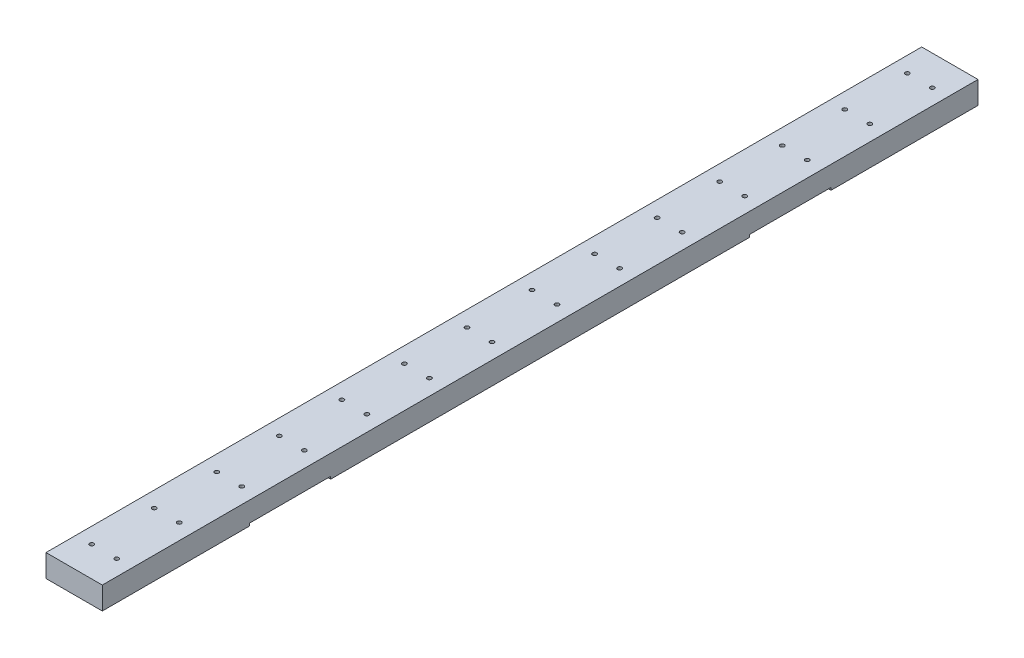
SolidWorks part; units mm, degrees
material "6061-T6"
ref_plane "Front Plane" through (0, 0, 0) normal (0, 0, 1) x (1, 0, 0)
ref_plane "Top Plane" through (0, 0, 0) normal (0, 1, 0) x (1, 0, 0)
ref_plane "Right Plane" through (0, 0, 0) normal (1, 0, 0) x (0, 0, -1)
sketch "Sketch1" plane through (0, 0, 0) normal (0, 0, 1) x (1, 0, 0)
  line L1 (-22.5, 9) -> (22.5, 9)
  line L2 (-22.5, 9) -> (-22.5, -9)
  line L3 (-22.5, -9) -> (22.5, -9)
  line L4 (22.5, 9) -> (22.5, -9)
  line L5 (-22.5, 9) -> (22.5, -9) construction
  line L6 (-22.5, -9) -> (22.5, 9) construction
  point P0 (0, 0)
  dimension "D1" = 45
  dimension "D2" = 18
extrude "Boss-Extrude1" add sketch "Sketch1" along normal mid plane 700
hole_wizard "M4 Tapped Hole1" positions "Sketch2" profile "Sketch3" tap size "M4" standard "GB"
sketch "Sketch2" plane through (-22.5, 0, 0) normal (-1, 0, 0) x (0, 0, 1)
  line L0 (-345, 0) -> (-350, 0)
  line L1 (-350, 9) -> (-350, -9) construction
  line L2 (-345, 0) -> (-300, 0)
  line L3 (300, 0) -> (345, 0)
  point P0 (-345, 0)
  point P19 (-300, 0)
  point P33 (-250, 0)
  point P34 (-200, 0)
  point P35 (-150, 0)
  point P36 (-100, 0)
  point P37 (-50, 0)
  point P38 (0, 0)
  point P39 (50, 0)
  point P40 (100, 0)
  point P41 (150, 0)
  point P42 (200, 0)
  point P43 (250, 0)
  point P44 (300, 0)
  point P46 (345, 0)
  dimension "D1" = 5
  dimension "D2" = 45
  dimension "D4" = 50
  dimension "D5" = 45
  dimension "D3" = 13
sketch "Sketch3" plane through (-22.5, 0, -345) normal (0, 1, 0) x (0, 0, 1)
  line L0 (0, 0) -> (0, 11.0914)
  line L1 (0, 11.0914) -> (1.65, 10.1)
  line L2 (1.65, 10.1) -> (1.65, 0)
  line L5 (1.65, 0) -> (0, 0)
  line L10 (0, 11.0914) -> (-1.65, 10.1) construction
  line L11 (0, -6.35) -> (0, 107.95) construction
  dimension "螺纹孔钻头直径" = 3.3
  dimension "螺纹孔钻头深度" = 10.1
  dimension "导头角度" = 118
cosmetic thread "Hole Thread1" parameters "D1"=8, "D2"=4
cosmetic thread "Hole Thread55" parameters "D1"=8, "D2"=4
cosmetic thread "Hole Thread56" parameters "D1"=8, "D2"=4
cosmetic thread "Hole Thread57" parameters "D1"=8, "D2"=4
cosmetic thread "Hole Thread58" parameters "D1"=8, "D2"=4
cosmetic thread "Hole Thread59" parameters "D1"=8, "D2"=4
cosmetic thread "Hole Thread60" parameters "D1"=8, "D2"=4
cosmetic thread "Hole Thread61" parameters "D1"=8, "D2"=4
cosmetic thread "Hole Thread62" parameters "D1"=8, "D2"=4
cosmetic thread "Hole Thread63" parameters "D1"=8, "D2"=4
cosmetic thread "Hole Thread64" parameters "D1"=8, "D2"=4
cosmetic thread "Hole Thread65" parameters "D1"=8, "D2"=4
cosmetic thread "Hole Thread66" parameters "D1"=8, "D2"=4
cosmetic thread "Hole Thread67" parameters "D1"=8, "D2"=4
cosmetic thread "Hole Thread68" parameters "D1"=8, "D2"=4
pattern_linear "LPattern1" count 14 spacing 50
cosmetic thread "Hole Thread2" parameters "D1"=8, "D2"=4
cosmetic thread "Hole Thread3" parameters "D1"=8, "D2"=4
cosmetic thread "Hole Thread4" parameters "D1"=8, "D2"=4
cosmetic thread "Hole Thread5" parameters "D1"=8, "D2"=4
cosmetic thread "Hole Thread6" parameters "D1"=8, "D2"=4
cosmetic thread "Hole Thread7" parameters "D1"=8, "D2"=4
cosmetic thread "Hole Thread8" parameters "D1"=8, "D2"=4
cosmetic thread "Hole Thread9" parameters "D1"=8, "D2"=4
cosmetic thread "Hole Thread10" parameters "D1"=8, "D2"=4
cosmetic thread "Hole Thread11" parameters "D1"=8, "D2"=4
cosmetic thread "Hole Thread12" parameters "D1"=8, "D2"=4
cosmetic thread "Hole Thread13" parameters "D1"=8, "D2"=4
cosmetic thread "Hole Thread14" parameters "D1"=8, "D2"=4
hole_wizard "M4 Tapped Hole3" positions "Sketch4" profile "Sketch5" tap size "M4" standard "GB" end condition through all
sketch "Sketch4" plane through (0, -9, 0) normal (0, -1, 0) x (-1, 0, 0)
  line L0 (10, -276) -> (10, -226)
  line L1 (10, -226) -> (-10, -226)
  line L2 (-10, -226) -> (-10, -176)
  line L3 (-10, -176) -> (10, -176)
  line L4 (10, -176) -> (10, -126)
  line L5 (10, -126) -> (-10, -126)
  line L6 (-10, -126) -> (-10, -76)
  line L7 (-10, -76) -> (10, -76)
  line L9 (10, -276) -> (-10, -276)
  line L10 (-10, -276) -> (-10, -226)
  line L12 (10, -226) -> (10, -176)
  line L14 (-10, -176) -> (-10, -126)
  line L16 (10, -126) -> (10, -76)
  line L18 (22.5, -350) -> (-22.5, -350) construction
  line L19 (22.5, -350) -> (22.5, 350) construction
  line L20 (10, -276) -> (10, -326)
  line L21 (10, -326) -> (-10, -326)
  line L22 (-10, -326) -> (-10, -276)
  line L23 (-10, 276) -> (10, 276)
  line L24 (10, 276) -> (10, 226)
  line L25 (10, 226) -> (-10, 226)
  line L26 (-10, 226) -> (-10, 176)
  line L27 (-10, 176) -> (10, 176)
  line L28 (10, 176) -> (10, 126)
  line L29 (10, 126) -> (-10, 126)
  line L30 (-10, 126) -> (-10, 76)
  line L31 (-10, 76) -> (10, 76)
  line L32 (10, 76) -> (10, 26)
  line L33 (10, 26) -> (-10, 26)
  line L34 (-10, 26) -> (-10, 0)
  line L35 (-10, 0) -> (10, 0)
  line L36 (10, 0) -> (10, -26)
  line L37 (10, -26) -> (-10, -26)
  line L38 (-10, -26) -> (-10, -76)
  line L40 (10, -76) -> (10, -26)
  line L42 (-10, -26) -> (-10, 0)
  line L44 (10, 0) -> (10, 26)
  line L46 (-10, 26) -> (-10, 76)
  line L48 (10, 76) -> (10, 126)
  line L50 (-10, 126) -> (-10, 176)
  line L52 (10, 176) -> (10, 226)
  line L54 (-10, 226) -> (-10, 276)
  line L56 (10, 276) -> (10, 326)
  line L57 (10, 326) -> (-10, 326)
  line L58 (-10, 326) -> (-10, 276)
  line L60 (22.5, 350) -> (-22.5, 350) construction
  point P4 (10, -176)
  point P6 (-10, -176)
  point P8 (10, -126)
  point P10 (-10, -126)
  point P16 (10, -226)
  point P18 (-10, -226)
  point P21 (10, -276)
  point P33 (-10, -76)
  point P35 (10, -76)
  point P39 (-10, -276)
  point P56 (0, -276)
  point P59 (10, -326)
  point P61 (-10, -326)
  point P93 (10, 176)
  point P95 (-10, 176)
  point P97 (10, 226)
  point P99 (-10, 226)
  point P105 (10, 326)
  point P107 (-10, 326)
  point P110 (-10, 276)
  point P111 (10, 276)
  point P119 (10, 126)
  point P121 (-10, 126)
  point P123 (-10, 76)
  point P124 (10, 76)
  point P126 (10, 26)
  point P128 (-10, 26)
  point P132 (10, -26)
  point P133 (-10, -26)
  dimension "D1" = 50
  dimension "D2" = 50
  dimension "D3" = 20
  dimension "D4" = 22.5
  dimension "D5" = 24
  dimension "D6" = 24
  dimension "D7" = 50
sketch "Sketch5" plane through (-10, -9, 176) normal (1, 0, 0) x (0, 0, -1)
  line L0 (0, 0) -> (0, 18)
  line L1 (0, 18) -> (1.65, 18)
  line L2 (1.65, 18) -> (1.65, 0)
  line L5 (1.65, 0) -> (0, 0)
  line L11 (0, -6.35) -> (0, 107.95) construction
  dimension "通孔螺纹孔钻头直径" = 3.3
  dimension "通孔螺纹孔钻头深度" = 18
cosmetic thread "Hole Thread23" parameters "D2"=4
cosmetic thread "Hole Thread24" parameters "D2"=4
cosmetic thread "Hole Thread25" parameters "D2"=4
cosmetic thread "Hole Thread26" parameters "D2"=4
cosmetic thread "Hole Thread27" parameters "D2"=4
cosmetic thread "Hole Thread28" parameters "D2"=4
cosmetic thread "Hole Thread29" parameters "D2"=4
cosmetic thread "Hole Thread30" parameters "D2"=4
cosmetic thread "Hole Thread31" parameters "D2"=4
cosmetic thread "Hole Thread32" parameters "D2"=4
cosmetic thread "Hole Thread33" parameters "D2"=4
cosmetic thread "Hole Thread34" parameters "D2"=4
cosmetic thread "Hole Thread35" parameters "D2"=4
cosmetic thread "Hole Thread36" parameters "D2"=4
cosmetic thread "Hole Thread37" parameters "D2"=4
cosmetic thread "Hole Thread38" parameters "D2"=4
cosmetic thread "Hole Thread39" parameters "D2"=4
cosmetic thread "Hole Thread40" parameters "D2"=4
cosmetic thread "Hole Thread41" parameters "D2"=4
cosmetic thread "Hole Thread42" parameters "D2"=4
cosmetic thread "Hole Thread43" parameters "D2"=4
cosmetic thread "Hole Thread44" parameters "D2"=4
cosmetic thread "Hole Thread45" parameters "D2"=4
cosmetic thread "Hole Thread46" parameters "D2"=4
cosmetic thread "Hole Thread47" parameters "D2"=4
cosmetic thread "Hole Thread48" parameters "D2"=4
cosmetic thread "Hole Thread49" parameters "D2"=4
cosmetic thread "Hole Thread50" parameters "D2"=4
sketch "Sketch10" plane through (0, -9, 0) normal (0, -1, 0) x (1, 0, 0)
  line L0 (22.5, 350) -> (22.5, -350) construction
  line L1 (22.5, 167.5) -> (-22.5, 167.5)
  line L2 (22.5, 167.5) -> (22.5, 232.5)
  line L3 (22.5, 232.5) -> (-22.5, 232.5)
  line L4 (-22.5, 167.5) -> (-22.5, 232.5)
  line L5 (10, 200) -> (22.5, 200) construction
  line L6 (0, 0) -> (58.5676, 0) construction
  line L7 (-22.5, -167.5) -> (-22.5, -232.5)
  line L8 (22.5, -232.5) -> (-22.5, -232.5)
  line L9 (22.5, -167.5) -> (22.5, -232.5)
  line L10 (22.5, -167.5) -> (-22.5, -167.5)
  dimension "D1" = 65
  dimension "D2" = 45
  dimension "D3" = 200
extrude "Cut-Extrude3" cut sketch "Sketch10" against normal blind 2
hole_wizard "M4 Tapped Hole2" positions "Sketch8" profile "Sketch9" tap size "M4" standard "GB"
sketch "Sketch8" plane through (0, -7, 0) normal (0, -1, 0) x (-1, 0, 0)
  line L0 (-10.5, -220) -> (-10.5, -180)
  line L1 (-10.5, -180) -> (9.5, -180)
  line L2 (9.5, -180) -> (9.5, -220)
  line L3 (9.5, -220) -> (-10.5, -220)
  line L5 (-10, -200) -> (-10.5, -200)
  line L7 (-22.5, -350) -> (-22.5, -232.5) construction
  line L8 (0, 0) -> (-66.4729, 0) construction
  line L10 (-10, 200) -> (-10.5, 200)
  line L11 (9.5, 220) -> (-10.5, 220)
  line L12 (9.5, 180) -> (9.5, 220)
  line L13 (-10.5, 180) -> (9.5, 180)
  line L14 (-10.5, 220) -> (-10.5, 180)
  point P0 (9.5, -220)
  point P2 (-10.5, -220)
  point P4 (-10.5, -180)
  point P6 (9.5, -180)
  point P30 (9.5, 180)
  point P31 (-10.5, 180)
  point P32 (-10.5, 220)
  point P33 (9.5, 220)
  dimension "D1" = 40
  dimension "D2" = 12
  dimension "D3" = 20
  dimension "D4" = 200
sketch "Sketch9" plane through (-9.5, -7, 220) normal (1, 0, 0) x (0, 0, -1)
  line L0 (0, 0) -> (0, 11.0914)
  line L1 (0, 11.0914) -> (1.65, 10.1)
  line L2 (1.65, 10.1) -> (1.65, 0)
  line L5 (1.65, 0) -> (0, 0)
  line L10 (0, 11.0914) -> (-1.65, 10.1) construction
  line L11 (0, -6.35) -> (0, 107.95) construction
  dimension "螺纹孔钻头直径" = 3.3
  dimension "螺纹孔钻头深度" = 10.1
  dimension "导头角度" = 118
cosmetic thread "Hole Thread15" parameters "D1"=8, "D2"=4
cosmetic thread "Hole Thread16" parameters "D1"=8, "D2"=4
cosmetic thread "Hole Thread21" parameters "D1"=8, "D2"=4
cosmetic thread "Hole Thread22" parameters "D1"=8, "D2"=4
cosmetic thread "Hole Thread51" parameters "D1"=8, "D2"=4
cosmetic thread "Hole Thread52" parameters "D1"=8, "D2"=4
cosmetic thread "Hole Thread53" parameters "D1"=8, "D2"=4
cosmetic thread "Hole Thread54" parameters "D1"=8, "D2"=4
